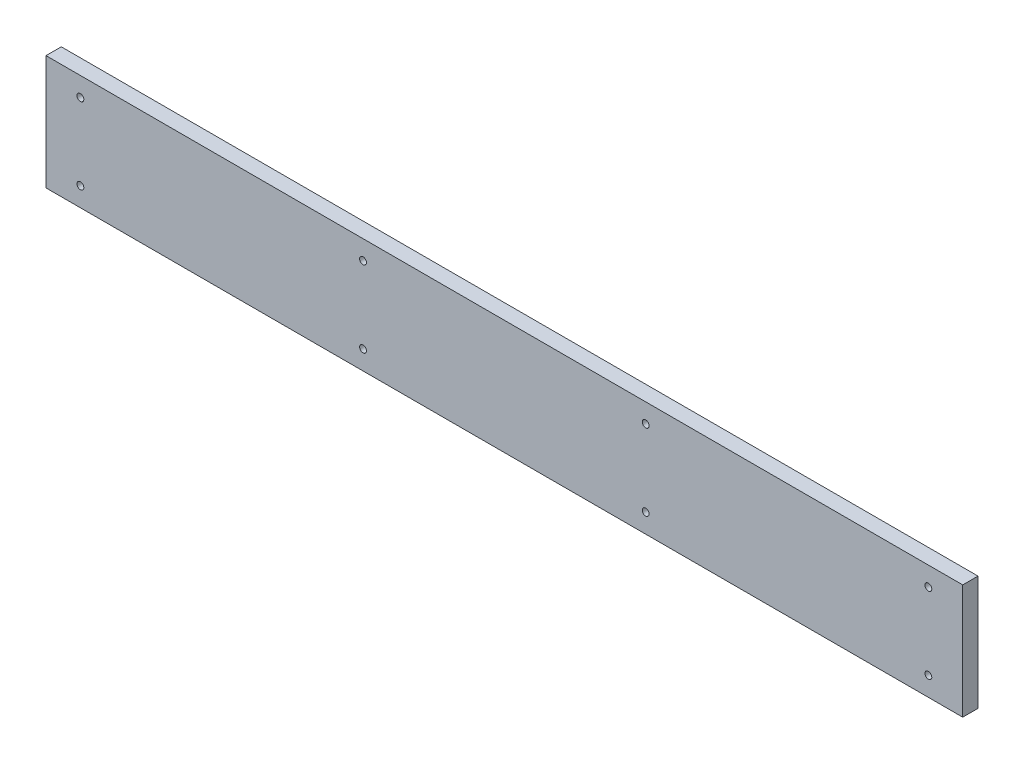
SolidWorks part; units mm, degrees
material "PUR"
ref_plane "Front Plane" through (0, 0, 0) normal (0, 0, 1) x (1, 0, 0)
ref_plane "Top Plane" through (0, 0, 0) normal (0, 1, 0) x (1, 0, 0)
ref_plane "Right Plane" through (0, 0, 0) normal (1, 0, 0) x (0, 0, -1)
sketch "Sketch1" plane through (0, 0, 0) normal (0, 0, 1) x (1, 0, 0)
  line L1 (1200, 0) -> (0, 0)
  line L2 (1200, 0) -> (1200, 150)
  line L3 (1200, 150) -> (0, 150)
  line L4 (0, 0) -> (0, 150)
  dimension "D1" = 1200
  dimension "D2" = 150
extrude "Boss-Extrude1" add sketch "Sketch1" along normal blind 20 contours L1 L4 L3 L2
hole_wizard "Hole size (by socket head cap screw type)1" positions "Sketch2" profile "Sketch3" counterbore size "M8" standard "GB" end condition through all
sketch "Sketch2" plane through (0, 0, 0) normal (0, 0, -1) x (-1, 0, 0)
  line L0 (-1155, 125) -> (-1155, 25) construction
  line L1 (-1155, 25) -> (-45, 25) construction
  line L2 (-45, 25) -> (-45, 125) construction
  line L3 (-45, 125) -> (-1155, 125) construction
  line L5 (-785, 125) -> (-785, 25) construction
  line L7 (-415, 125) -> (-415, 25) construction
  line L9 (-1200, 0) -> (-1200, 150) construction
  line L10 (0, 0) -> (0, 150) construction
  line L11 (-1200, 150) -> (0, 150) construction
  line L12 (-1200, 0) -> (0, 0) construction
  point P0 (-1155, 125)
  point P2 (-1155, 25)
  point P4 (-785, 25)
  point P6 (-415, 25)
  point P8 (-45, 25)
  point P10 (-45, 125)
  point P12 (-415, 125)
  point P14 (-785, 125)
  dimension "D1" = 45
  dimension "D2" = 45
  dimension "D3" = 25
  dimension "D4" = 25
  dimension "D5" = 370
  dimension "D6" = 370
sketch "Sketch3" plane through (1155, 125, 0) normal (1, 0, 0) x (0, 1, 0)
  line L0 (0, 0) -> (0, 20)
  line L1 (0, 20) -> (4.5, 20)
  line L3 (4.5, 20) -> (4.5, 9)
  line L4 (4.5, 9) -> (7.5, 9)
  line L5 (7.5, 9) -> (7.5, 0)
  line L7 (7.5, 0) -> (0, 0)
  line L11 (0, -6.35) -> (0, 107.95) construction
  dimension "通孔孔直径" = 9
  dimension "通孔孔深度" = 20
  dimension "柱形沉头孔直径" = 15
  dimension "柱形沉头孔深度" = 9
sketch "Sketch4" plane through (0, 0, 0) normal (0, 0, -1) x (-1, 0, 0)
  line L0 (-1200, 0) -> (0, 0) construction
  line L1 (0, 0) -> (0, 150) construction
  circle A0 centre (-50, 30) radius 22.5
  circle A1 centre (-50, 30) radius 19.5
  dimension "D1" = 45
  dimension "D2" = 39
  dimension "D3" = 30
  dimension "D4" = 50
extrude "Cut-Extrude1" cut sketch "Sketch4" against normal blind 3
pattern_linear "LPattern1" count 4 spacing 30 along (0, 1, 0) of "Cut-Extrude1"
pattern_linear "LPattern2" count 23 spacing 50 along (1, 0, 0) of "LPattern1", "Cut-Extrude1"
